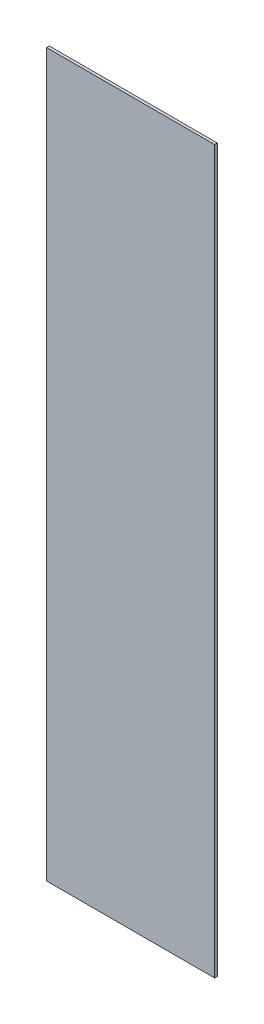
from build123d import *

# Parameters (mm, degrees)
SKETCH_1_W      = 304
SKETCH_1_H      = 1306
EXTRUDE_1_DEPTH = 5


with BuildPart() as part:
    # 草图1 → 凸台-拉伸1 (new body)
    with BuildSketch(Plane.XY):
        Rectangle(SKETCH_1_W, SKETCH_1_H)
    extrude(amount=EXTRUDE_1_DEPTH)


solid = part.part
